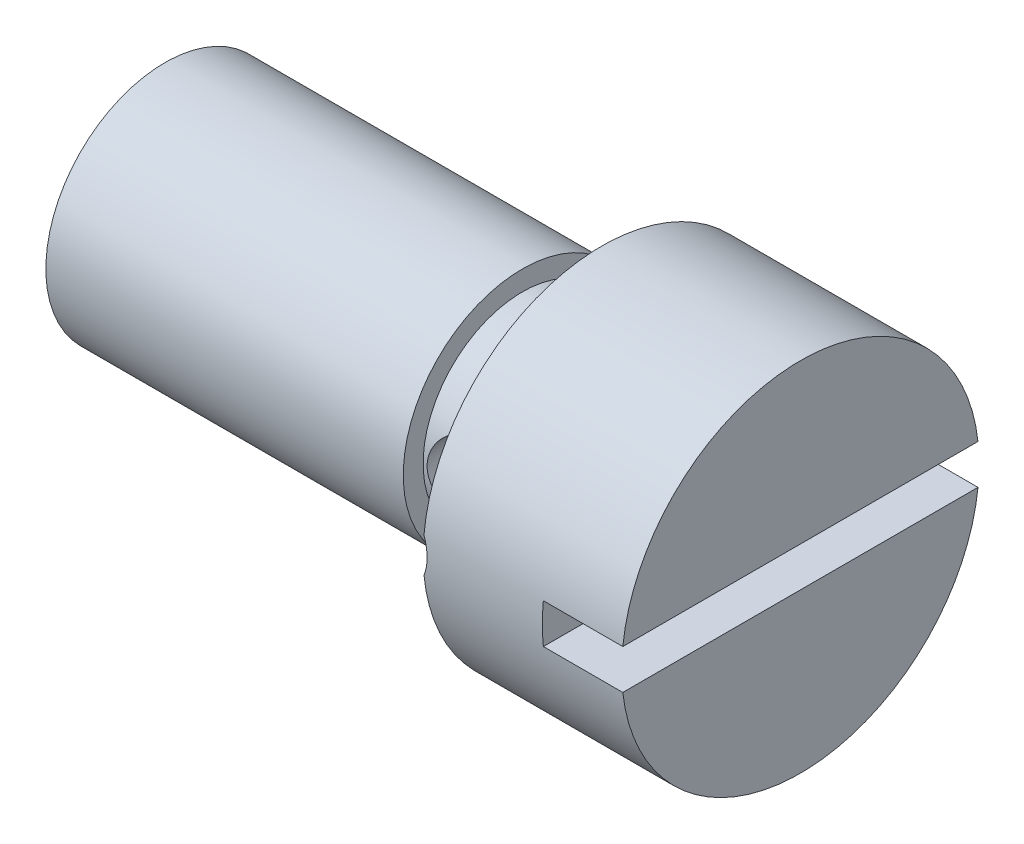
SolidWorks part; units mm, degrees
ref_plane "Front Plane" through (0, 0, 0) normal (0, 0, 1) x (1, 0, 0)
ref_plane "Top Plane" through (0, 0, 0) normal (0, 1, 0) x (1, 0, 0)
ref_plane "Right Plane" through (0, 0, 0) normal (1, 0, 0) x (0, 0, -1)
other "Configuration Table"
sketch "Sketch1" plane through (0, 0, 0) normal (1, 0, 0) x (0, 0, -1)
  circle A0 centre (0, 0) radius 3
  dimension "D1" = 6
extrude "Boss-Extrude1" add sketch "Sketch1" along normal blind 9
sketch "Sketch2" plane through (9, 0, 0) normal (1, 0, 0) x (0, 0, -1)
  circle A0 centre (0, 0) radius 2.5
  dimension "D1" = 5
extrude "Boss-Extrude2" add sketch "Sketch2" along normal blind 2
sketch "Sketch3" plane through (11, 0, 0) normal (1, 0, 0) x (0, 0, -1)
  circle A0 centre (0, 0) radius 4.5
  dimension "D1" = 9
extrude "Boss-Extrude3" add sketch "Sketch3" along normal blind 5
sketch "Sketch4" plane through (0, 0, 0) normal (-1, 0, 0) x (0, 0, 1)
  circle A0 centre (0, 0) radius 1
  dimension "D1" = 2
extrude "Cut-Extrude1" cut sketch "Sketch4" against normal blind 10.1 and the other way through all
sketch "Sketch6" plane through (0, 0, 0) normal (0, 0, 1) x (1, 0, 0)
  line L0 (10.1, 1) -> (10.1, -1) construction
  circle A0 centre (10.1, 0) radius 1
  dimension "D1" = 2
extrude "Cut-Extrude2" cut sketch "Sketch6" against normal through all both and the other way through all
sketch "Sketch7" plane through (0, 0, 0) normal (0, 0, 1) x (1, 0, 0)
  line L0 (16, -4.5) -> (16, 4.5) construction
  line L1 (14, 0.5) -> (18, 0.5)
  line L2 (14, 0.5) -> (14, -0.5)
  line L3 (14, -0.5) -> (18, -0.5)
  line L4 (18, 0.5) -> (18, -0.5)
  line L5 (14, 0.5) -> (18, -0.5) construction
  line L6 (14, -0.5) -> (18, 0.5) construction
  point P0 (16, 0)
  dimension "D1" = 1
  dimension "D2" = 4
extrude "Cut-Extrude3" cut sketch "Sketch7" against normal through all both and the other way through all
